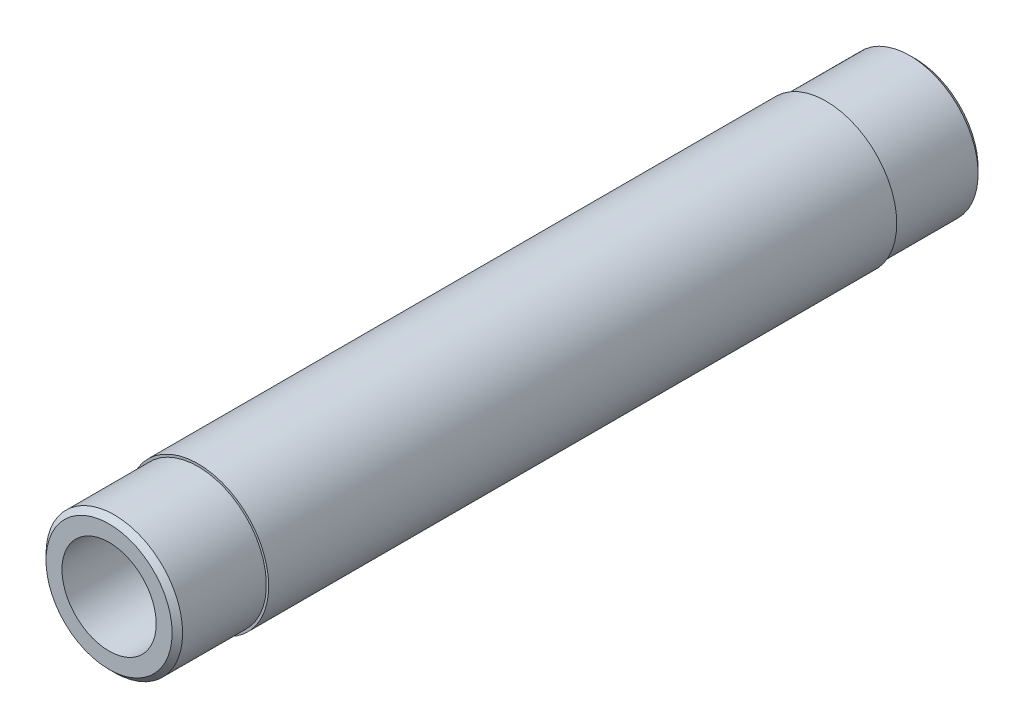
SolidWorks part; units mm, degrees
material "黄铜"
ref_plane "前视基准面" through (0, 0, 0) normal (0, 0, 1) x (1, 0, 0)
ref_plane "上视基准面" through (0, 0, 0) normal (0, 1, 0) x (1, 0, 0)
ref_plane "右视基准面" through (0, 0, 0) normal (1, 0, 0) x (0, 0, -1)
sketch "草图1" plane through (0, 0, 0) normal (0, 0, 1) x (1, 0, 0)
  line L0 (-1000, 0) -> (49000, 0) construction
  line L1 (15.5885, 0) -> (7.7942, 13.5) construction
  line L2 (7.7942, 13.5) -> (-7.7942, 13.5) construction
  line L3 (-7.7942, 13.5) -> (-15.5885, 0) construction
  line L4 (-15.5885, 0) -> (-7.7942, -13.5) construction
  line L5 (-7.7942, -13.5) -> (7.7942, -13.5) construction
  line L6 (7.7942, -13.5) -> (15.5885, 0) construction
  circle A0 centre (0, 0) radius 13.5
  dimension "D1" = 27
extrude "凸台-拉伸1" add sketch "草图1" along normal mid plane 120
sketch "草图4" plane through (0, 0, -60) normal (0, 0, -1) x (-1, 0, 0)
  circle A0 centre (0, 0) radius 13.05
  dimension "D1" = 26.1
extrude "凸台-拉伸3" add sketch "草图4" along normal blind 17
cosmetic thread "装饰螺纹线2" parameters "D2"=18.631
mirror "镜向1" about plane through (0, 0, 0) normal (0, 0, 1) of "凸台-拉伸3"
sketch "草图5" plane through (0, 0, -77) normal (0, 0, -1) x (-1, 0, 0)
  circle A0 centre (0, 0) radius 9
  dimension "D1" = 18
extrude "切除-拉伸2" cut sketch "草图5" against normal up to next
chamfer "倒角1" distance 1 angle 45 2 edges at (-13.05, 0, -77) (-13.05, 0, 77)
